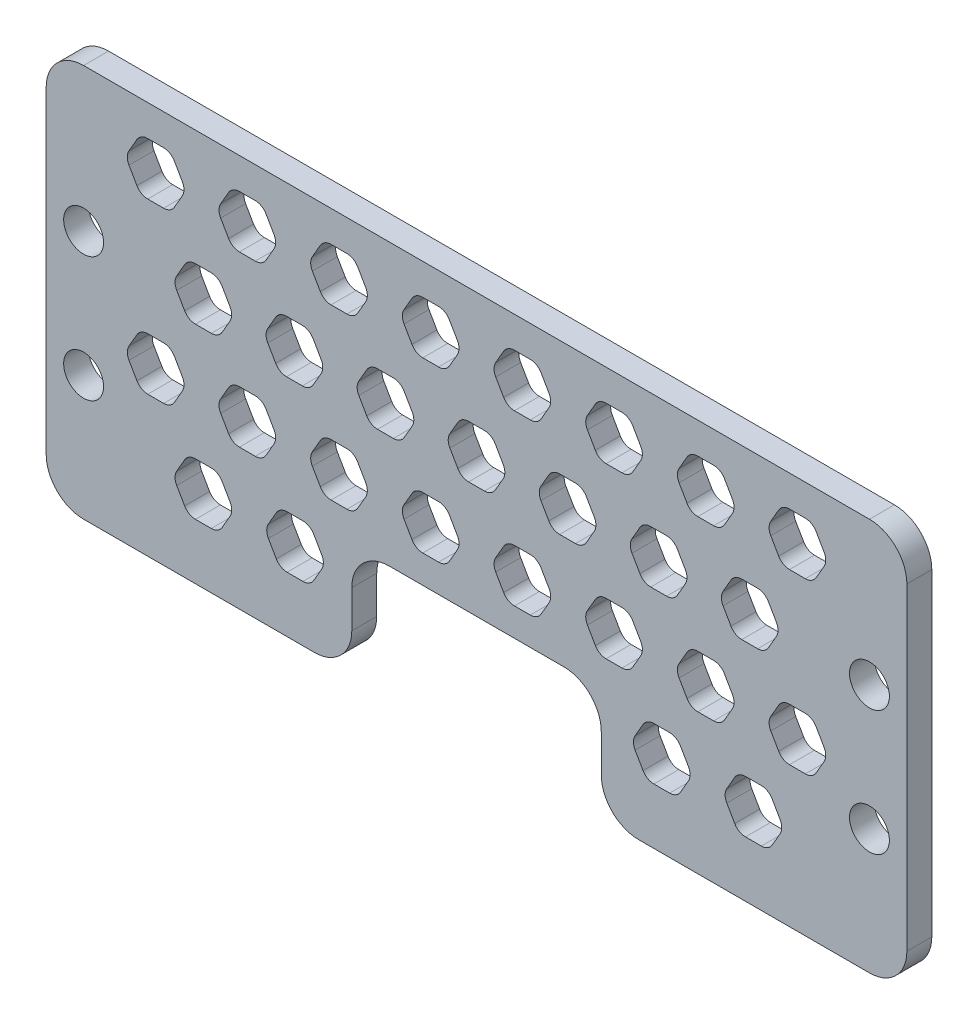
from build123d import *

# Parameters (mm, degrees)
SKETCH_1_R          = 1.6
EXTRUDE_1_DEPTH     = 2
CUT_EXTRUDE_1_DEPTH = 38.977789562
FILLET_R1_R         = 1
FILLET_R3_R         = 3


with BuildPart() as part:
    # 草图1 → 凸台-拉伸1 (new body)
    with BuildSketch(Plane.XY):
        Polygon((-34.5, 15.75), (34.5, 15.75), (34.5, -15.75), (10, -15.75), (10, -6.75), (-10, -6.75), (-10, -15.75), (-34.5, -15.75), align=None)
        with Locations((-31.5, 4.25)):
            Circle(SKETCH_1_R, mode=Mode.SUBTRACT)
        with Locations((-31.5, -5.75)):
            Circle(SKETCH_1_R, mode=Mode.SUBTRACT)
        with Locations(Location((31.5, -5.75, 0), (0, 0, 180))):
            Circle(SKETCH_1_R, mode=Mode.SUBTRACT)
        with Locations(Location((31.5, 4.25, 0), (0, 0, 180))):
            Circle(SKETCH_1_R, mode=Mode.SUBTRACT)
    extrude(amount=EXTRUDE_1_DEPTH)

    # 草图2 → 切除-拉伸1 (cut, through all)
    with BuildSketch(Plane.XY.offset(2)):
        Polygon((-28.148969045, 11.15), (-26.936533479, 13.25), (-24.511662349, 13.25), (-23.299226784, 11.15), (-24.511662349, 9.05), (-26.936533479, 9.05), align=None)
        Polygon((-19.586791218, 9.05), (-20.799226784, 11.15), (-19.586791218, 13.25), (-17.161920088, 13.25), (-15.949484522, 11.15), (-17.161920088, 9.05), align=None)
        Polygon((-12.237048957, 9.05), (-13.449484522, 11.15), (-12.237048957, 13.25), (-9.812177826, 13.25), (-8.599742261, 11.15), (-9.812177826, 9.05), align=None)
        Polygon((-4.887306696, 9.05), (-6.099742261, 11.15), (-4.887306696, 13.25), (-2.462435565, 13.25), (-1.25, 11.15), (-2.462435565, 9.05), align=None)
        Polygon((2.462435565, 9.05), (1.25, 11.15), (2.462435565, 13.25), (4.887306696, 13.25), (6.099742261, 11.15), (4.887306696, 9.05), align=None)
        Polygon((9.812177826, 9.05), (8.599742261, 11.15), (9.812177826, 13.25), (12.237048957, 13.25), (13.449484522, 11.15), (12.237048957, 9.05), align=None)
        Polygon((17.161920088, 9.05), (15.949484522, 11.15), (17.161920088, 13.25), (19.586791218, 13.25), (20.799226784, 11.15), (19.586791218, 9.05), align=None)
        Polygon((24.511662349, 9.05), (23.299226784, 11.15), (24.511662349, 13.25), (26.936533479, 13.25), (28.148969045, 11.15), (26.936533479, 9.05), align=None)
        Polygon((-24.324097914, 4.374871131), (-23.111662349, 6.474871131), (-20.686791218, 6.474871131), (-19.474355653, 4.374871131), (-20.686791218, 2.274871131), (-23.111662349, 2.274871131), align=None)
        Polygon((-15.811920088, 2.274871131), (-17.024355653, 4.374871131), (-15.811920088, 6.474871131), (-13.387048957, 6.474871131), (-12.174613392, 4.374871131), (-13.387048957, 2.274871131), align=None)
        Polygon((-8.512177826, 2.274871131), (-9.724613392, 4.374871131), (-8.512177826, 6.474871131), (-6.087306696, 6.474871131), (-4.874871131, 4.374871131), (-6.087306696, 2.274871131), align=None)
        Polygon((-1.212435565, 2.274871131), (-2.424871131, 4.374871131), (-1.212435565, 6.474871131), (1.212435565, 6.474871131), (2.424871131, 4.374871131), (1.212435565, 2.274871131), align=None)
        Polygon((6.087306696, 2.274871131), (4.874871131, 4.374871131), (6.087306696, 6.474871131), (8.512177826, 6.474871131), (9.724613392, 4.374871131), (8.512177826, 2.274871131), align=None)
        Polygon((13.387048957, 2.274871131), (12.174613392, 4.374871131), (13.387048957, 6.474871131), (15.811920088, 6.474871131), (17.024355653, 4.374871131), (15.811920088, 2.274871131), align=None)
        Polygon((20.686791218, 2.274871131), (19.474355653, 4.374871131), (20.686791218, 6.474871131), (23.111662349, 6.474871131), (24.324097914, 4.374871131), (23.111662349, 2.274871131), align=None)
        Polygon((-26.936533479, -4.500257739), (-28.148969045, -2.400257739), (-26.936533479, -0.300257739), (-24.511662349, -0.300257739), (-23.299226784, -2.400257739), (-24.511662349, -4.500257739), align=None)
        Polygon((-19.586791218, -4.500257739), (-20.799226784, -2.400257739), (-19.586791218, -0.300257739), (-17.161920088, -0.300257739), (-15.949484522, -2.400257739), (-17.161920088, -4.500257739), align=None)
        Polygon((-12.237048957, -4.500257739), (-13.449484522, -2.400257739), (-12.237048957, -0.300257739), (-9.812177826, -0.300257739), (-8.599742261, -2.400257739), (-9.812177826, -4.500257739), align=None)
        Polygon((-4.887306696, -4.500257739), (-6.099742261, -2.400257739), (-4.887306696, -0.300257739), (-2.462435565, -0.300257739), (-1.25, -2.400257739), (-2.462435565, -4.500257739), align=None)
        Polygon((2.462435565, -4.500257739), (1.25, -2.400257739), (2.462435565, -0.300257739), (4.887306696, -0.300257739), (6.099742261, -2.400257739), (4.887306696, -4.500257739), align=None)
        Polygon((9.812177826, -4.500257739), (8.599742261, -2.400257739), (9.812177826, -0.300257739), (12.237048957, -0.300257739), (13.449484522, -2.400257739), (12.237048957, -4.500257739), align=None)
        Polygon((17.161920088, -4.500257739), (15.949484522, -2.400257739), (17.161920088, -0.300257739), (19.586791218, -0.300257739), (20.799226784, -2.400257739), (19.586791218, -4.500257739), align=None)
        Polygon((24.511662349, -4.500257739), (23.299226784, -2.400257739), (24.511662349, -0.300257739), (26.936533479, -0.300257739), (28.148969045, -2.400257739), (26.936533479, -4.500257739), align=None)
        Polygon((-24.324097914, -9.175386608), (-23.111662349, -7.075386608), (-20.686791218, -7.075386608), (-19.474355653, -9.175386608), (-20.686791218, -11.275386608), (-23.111662349, -11.275386608), align=None)
        Polygon((-15.761920088, -11.275386608), (-16.974355653, -9.175386608), (-15.761920088, -7.075386608), (-13.337048957, -7.075386608), (-12.124613392, -9.175386608), (-13.337048957, -11.275386608), align=None)
        Polygon((13.637048957, -11.275386608), (12.424613392, -9.175386608), (13.637048957, -7.075386608), (16.061920088, -7.075386608), (17.274355653, -9.175386608), (16.061920088, -11.275386608), align=None)
        Polygon((20.986791218, -11.275386608), (19.774355653, -9.175386608), (20.986791218, -7.075386608), (23.411662349, -7.075386608), (24.624097914, -9.175386608), (23.411662349, -11.275386608), align=None)
    extrude(amount=-CUT_EXTRUDE_1_DEPTH, mode=Mode.SUBTRACT)

    # R1 镂空圆角
    fillet_r1_edges = [part.edges().sort_by_distance(p)[0] for p in [
        (-28.148969045, -2.400257739, 1),
        (-26.936533479, -0.300257739, 1),
        (-24.511662349, -0.300257739, 1),
        (-23.299226784, -2.400257739, 1),
        (-24.511662349, -4.500257739, 1),
        (-26.936533479, -4.500257739, 1),
        (-17.024355653, 4.374871131, 1),
        (-15.811920088, 6.474871131, 1),
        (-13.387048957, 6.474871131, 1),
        (-12.174613392, 4.374871131, 1),
        (-13.387048957, 2.274871131, 1),
        (-15.811920088, 2.274871131, 1),
        (-9.724613392, 4.374871131, 1),
        (-8.512177826, 6.474871131, 1),
        (-6.087306696, 6.474871131, 1),
        (-4.874871131, 4.374871131, 1),
        (-6.087306696, 2.274871131, 1),
        (-8.512177826, 2.274871131, 1),
        (-2.424871131, 4.374871131, 1),
        (-1.212435565, 6.474871131, 1),
        (1.212435565, 6.474871131, 1),
        (2.424871131, 4.374871131, 1),
        (1.212435565, 2.274871131, 1),
        (-1.212435565, 2.274871131, 1),
        (-20.799226784, -2.400257739, 1),
        (-19.586791218, -0.300257739, 1),
        (-17.161920088, -0.300257739, 1),
        (-15.949484522, -2.400257739, 1),
        (-17.161920088, -4.500257739, 1),
        (-19.586791218, -4.500257739, 1),
        (19.474355653, 4.374871131, 1),
        (20.686791218, 6.474871131, 1),
        (23.111662349, 6.474871131, 1),
        (24.324097914, 4.374871131, 1),
        (23.111662349, 2.274871131, 1),
        (20.686791218, 2.274871131, 1),
        (12.174613392, 4.374871131, 1),
        (13.387048957, 6.474871131, 1),
        (15.811920088, 6.474871131, 1),
        (17.024355653, 4.374871131, 1),
        (15.811920088, 2.274871131, 1),
        (13.387048957, 2.274871131, 1),
        (4.874871131, 4.374871131, 1),
        (6.087306696, 6.474871131, 1),
        (8.512177826, 6.474871131, 1),
        (9.724613392, 4.374871131, 1),
        (8.512177826, 2.274871131, 1),
        (6.087306696, 2.274871131, 1),
        (-20.799226784, 11.15, 1),
        (-19.586791218, 13.25, 1),
        (-17.161920088, 13.25, 1),
        (-15.949484522, 11.15, 1),
        (-17.161920088, 9.05, 1),
        (-19.586791218, 9.05, 1),
        (-13.449484522, 11.15, 1),
        (-12.237048957, 13.25, 1),
        (-9.812177826, 13.25, 1),
        (-8.599742261, 11.15, 1),
        (-9.812177826, 9.05, 1),
        (-12.237048957, 9.05, 1),
        (-6.099742261, 11.15, 1),
        (-4.887306696, 13.25, 1),
        (-2.462435565, 13.25, 1),
        (-1.25, 11.15, 1),
        (-2.462435565, 9.05, 1),
        (-4.887306696, 9.05, 1),
        (1.25, 11.15, 1),
        (2.462435565, 13.25, 1),
        (4.887306696, 13.25, 1),
        (6.099742261, 11.15, 1),
        (4.887306696, 9.05, 1),
        (2.462435565, 9.05, 1),
        (-23.111662349, 2.274871131, 1),
        (-24.324097914, 4.374871131, 1),
        (-23.111662349, 6.474871131, 1),
        (-20.686791218, 6.474871131, 1),
        (-19.474355653, 4.374871131, 1),
        (-20.686791218, 2.274871131, 1),
        (23.299226784, 11.15, 1),
        (24.511662349, 13.25, 1),
        (26.936533479, 13.25, 1),
        (28.148969045, 11.15, 1),
        (26.936533479, 9.05, 1),
        (24.511662349, 9.05, 1),
        (15.949484522, 11.15, 1),
        (17.161920088, 13.25, 1),
        (19.586791218, 13.25, 1),
        (20.799226784, 11.15, 1),
        (19.586791218, 9.05, 1),
        (17.161920088, 9.05, 1),
        (8.599742261, 11.15, 1),
        (9.812177826, 13.25, 1),
        (12.237048957, 13.25, 1),
        (13.449484522, 11.15, 1),
        (12.237048957, 9.05, 1),
        (9.812177826, 9.05, 1),
        (19.774355653, -9.175386608, 1),
        (20.986791218, -7.075386608, 1),
        (23.411662349, -7.075386608, 1),
        (24.624097914, -9.175386608, 1),
        (23.411662349, -11.275386608, 1),
        (20.986791218, -11.275386608, 1),
        (12.424613392, -9.175386608, 1),
        (13.637048957, -7.075386608, 1),
        (16.061920088, -7.075386608, 1),
        (17.274355653, -9.175386608, 1),
        (16.061920088, -11.275386608, 1),
        (13.637048957, -11.275386608, 1),
        (-13.449484522, -2.400257739, 1),
        (-12.237048957, -0.300257739, 1),
        (-9.812177826, -0.300257739, 1),
        (-8.599742261, -2.400257739, 1),
        (-9.812177826, -4.500257739, 1),
        (-12.237048957, -4.500257739, 1),
        (-6.099742261, -2.400257739, 1),
        (-4.887306696, -0.300257739, 1),
        (-2.462435565, -0.300257739, 1),
        (-1.25, -2.400257739, 1),
        (-2.462435565, -4.500257739, 1),
        (-4.887306696, -4.500257739, 1),
        (1.25, -2.400257739, 1),
        (2.462435565, -0.300257739, 1),
        (4.887306696, -0.300257739, 1),
        (6.099742261, -2.400257739, 1),
        (4.887306696, -4.500257739, 1),
        (2.462435565, -4.500257739, 1),
        (8.599742261, -2.400257739, 1),
        (9.812177826, -0.300257739, 1),
        (12.237048957, -0.300257739, 1),
        (13.449484522, -2.400257739, 1),
        (12.237048957, -4.500257739, 1),
        (9.812177826, -4.500257739, 1),
        (15.949484522, -2.400257739, 1),
        (17.161920088, -0.300257739, 1),
        (19.586791218, -0.300257739, 1),
        (20.799226784, -2.400257739, 1),
        (19.586791218, -4.500257739, 1),
        (17.161920088, -4.500257739, 1),
        (23.299226784, -2.400257739, 1),
        (24.511662349, -0.300257739, 1),
        (26.936533479, -0.300257739, 1),
        (28.148969045, -2.400257739, 1),
        (26.936533479, -4.500257739, 1),
        (24.511662349, -4.500257739, 1),
        (-23.111662349, -11.275386608, 1),
        (-24.324097914, -9.175386608, 1),
        (-23.111662349, -7.075386608, 1),
        (-20.686791218, -7.075386608, 1),
        (-19.474355653, -9.175386608, 1),
        (-20.686791218, -11.275386608, 1),
        (-16.974355653, -9.175386608, 1),
        (-15.761920088, -7.075386608, 1),
        (-13.337048957, -7.075386608, 1),
        (-12.124613392, -9.175386608, 1),
        (-13.337048957, -11.275386608, 1),
        (-15.761920088, -11.275386608, 1),
        (-26.936533479, 9.05, 1),
        (-28.148969045, 11.15, 1),
        (-26.936533479, 13.25, 1),
        (-24.511662349, 13.25, 1),
        (-23.299226784, 11.15, 1),
        (-24.511662349, 9.05, 1),
    ]]
    fillet(fillet_r1_edges, radius=FILLET_R1_R)

    # R3 外缘圆角
    fillet_r3_edges = [part.edges().sort_by_distance(p)[0] for p in [
        (10, -15.75, 1),
        (10, -6.75, 1),
        (-10, -6.75, 1),
        (-10, -15.75, 1),
        (-34.5, -15.75, 1),
        (-34.5, 15.75, 1),
        (34.5, 15.75, 1),
        (34.5, -15.75, 1),
    ]]
    fillet(fillet_r3_edges, radius=FILLET_R3_R)


solid = part.part
